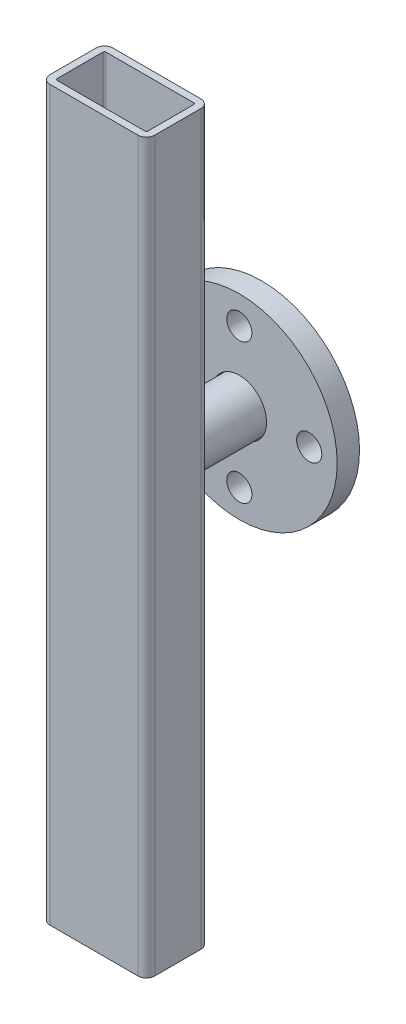
from build123d import *

# Parameters (mm, degrees)
EXTRUDE_1_DEPTH     = 521
SKETCH_2_R          = 19
EXTRUDE_2_DEPTH     = 75
SKETCH_3_R          = 70
SKETCH_3_R_2        = 9
EXTRUDE_3_DEPTH     = 16
SKETCH_4_R          = 39
EXTRUDE_4_DEPTH     = 2
CUT_EXTRUDE_START   = -77
SKETCH_5_R          = 19.5
SKETCH_5_R_2        = 19
CUT_EXTRUDE_1_DEPTH = 77


with BuildPart() as part:
    # 草图1 → 凸台-拉伸1 (new body)
    with BuildSketch(Plane(origin=(0, 0, 0), x_dir=(1, 0, 0), z_dir=(0, 1, 0))):
        with BuildLine():
            Line((-44, -7.278106509), (19, -7.278106509))
            ThreePointArc((19, -7.278106509), (23.242640687, -5.520747196), (25, -1.278106509))
            Line((25, -1.278106509), (25, 31.721893491))
            ThreePointArc((25, 31.721893491), (23.242640687, 35.964534178), (19, 37.721893491))
            Line((19, 37.721893491), (-44, 37.721893491))
            ThreePointArc((-44, 37.721893491), (-48.242640687, 35.964534178), (-50, 31.721893491))
            Line((-50, 31.721893491), (-50, -1.278106509))
            ThreePointArc((-50, -1.278106509), (-48.242640687, -5.520747196), (-44, -7.278106509))
        make_face()
        with BuildLine():
            Line((-44, -2.278106509), (19, -2.278106509))
            ThreePointArc((19, -2.278106509), (19.707106781, -1.98521329), (20, -1.278106509))
            Line((20, -1.278106509), (20, 31.721893491))
            ThreePointArc((20, 31.721893491), (19.707106781, 32.429000272), (19, 32.721893491))
            Line((19, 32.721893491), (-44, 32.721893491))
            ThreePointArc((-44, 32.721893491), (-44.707106781, 32.429000272), (-45, 31.721893491))
            Line((-45, 31.721893491), (-45, -1.278106509))
            ThreePointArc((-45, -1.278106509), (-44.707106781, -1.98521329), (-44, -2.278106509))
        make_face(mode=Mode.SUBTRACT)
    extrude(amount=EXTRUDE_1_DEPTH)

    # 草图2 → 凸台-拉伸2 (add)
    with BuildSketch(Plane(origin=(0, 0, -37.721893491), x_dir=(-1, 0, 0), z_dir=(0, 0, -1))):
        with Locations(Location((12.5, 285, 0), (0, 0, 180))):
            Circle(SKETCH_2_R)
    extrude(amount=EXTRUDE_2_DEPTH)

    # 草图3 → 凸台-拉伸3 (add)
    with BuildSketch(Plane(origin=(0, 0, -112.721893491), x_dir=(-1, 0, 0), z_dir=(0, 0, -1))):
        with Locations((12.5, 285)):
            Circle(SKETCH_3_R)
        with Locations((12.5, 335)):
            Circle(SKETCH_3_R_2, mode=Mode.SUBTRACT)
        with Locations((62.5, 285)):
            Circle(SKETCH_3_R_2, mode=Mode.SUBTRACT)
        with Locations((12.5, 235)):
            Circle(SKETCH_3_R_2, mode=Mode.SUBTRACT)
        with Locations((-37.5, 285)):
            Circle(SKETCH_3_R_2, mode=Mode.SUBTRACT)
    extrude(amount=-EXTRUDE_3_DEPTH)

    # 草图4 → 凸台-拉伸4 (add)
    with BuildSketch(Plane(origin=(0, 0, -112.721893491), x_dir=(-1, 0, 0), z_dir=(0, 0, -1))):
        with Locations((12.5, 285)):
            Circle(SKETCH_4_R)
    extrude(amount=EXTRUDE_4_DEPTH)

    # 草图5 → 切除-拉伸1 (cut)
    with BuildSketch(Plane(origin=(0, 0, -114.721893491), x_dir=(-1, 0, 0), z_dir=(0, 0, -1)).offset(CUT_EXTRUDE_START)):
        with Locations((12.5, 285)):
            Circle(SKETCH_5_R)
        with Locations(Location((12.5, 285, 0), (0, 0, 180))):
            Circle(SKETCH_5_R_2, mode=Mode.SUBTRACT)
    extrude(amount=CUT_EXTRUDE_1_DEPTH, mode=Mode.SUBTRACT)


with BuildPart() as cut_extrude_1_piece_1:
    # of the separate pieces the step leaves, piece 1, a body of its own (cut_extrude_1_pieces)
    add(part.part.solids().sort_by_distance((-44, 0, 7.278106509))[0])


with BuildPart() as cut_extrude_1_piece_2:
    # of the separate pieces the step leaves, piece 2, a body of its own (cut_extrude_1_pieces)
    add(part.part.solids().sort_by_distance((-82.5, 285, -96.721893491))[0])


solid = Compound([cut_extrude_1_piece_1.part, cut_extrude_1_piece_2.part])
